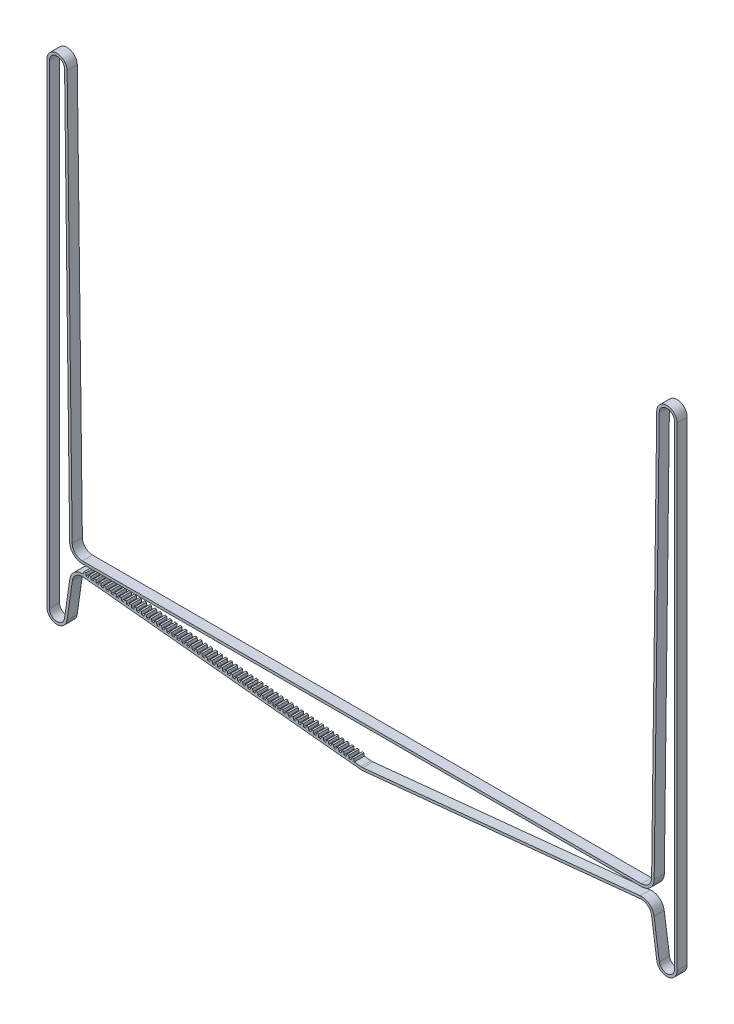
from build123d import *

# Parameters (mm, degrees)
BOSS_EXTRUDE1_DEPTH = 6
BOSS_EXTRUDE2_DEPTH = 6
LPATTERN1_COUNT     = 54
LPATTERN1_PITCH     = 3


with BuildPart() as part:
    # Sketch1 → Boss-Extrude1 (new body)
    with BuildSketch(Plane.XY):
        with BuildLine():
            Line((-136.619529898, -129.381794908), (27.031698215, -145.814248682))
            ThreePointArc((27.031698215, -145.814248682), (27.78101593, -145.851774363), (28.530333645, -145.814248682))
            Line((28.530333645, -145.814248682), (192.181561758, -129.381794908))
            ThreePointArc((192.181561758, -129.381794908), (196.478349535, -130.626340604), (198.719904672, -134.497607806))
            Line((198.719904672, -134.497607806), (201.842127188, -156.20594092))
            ThreePointArc((201.842127188, -156.20594092), (208.209190863, -161.336477048), (213.78101593, -155.351774363))
            Line((213.78101593, -155.351774363), (213.78101593, 124.648225637))
            ThreePointArc((213.78101593, 124.648225637), (207.818502024, 130.648108535), (201.781484333, 124.723196362))
            Line((201.781484333, 124.723196362), (198.780547528, -115.426745088))
            ThreePointArc((198.780547528, -115.426745088), (196.997067143, -119.620838918), (192.78101593, -121.351774363))
            Line((192.78101593, -121.351774363), (-137.21898407, -121.351774363))
            ThreePointArc((-137.21898407, -121.351774363), (-141.435035282, -119.620838918), (-143.218515667, -115.426745088))
            Line((-143.218515667, -115.426745088), (-146.219452472, 124.723196362))
            ThreePointArc((-146.219452472, 124.723196362), (-152.256470164, 130.648108535), (-158.21898407, 124.648225637))
            Line((-158.21898407, 124.648225637), (-158.21898407, -155.351774363))
            ThreePointArc((-158.21898407, -155.351774363), (-152.647159003, -161.336477048), (-146.280095328, -156.20594092))
            Line((-146.280095328, -156.20594092), (-143.157872812, -134.497607806))
            ThreePointArc((-143.157872812, -134.497607806), (-140.916317675, -130.626340604), (-136.619529898, -129.381794908))
        make_face()
        with BuildLine():
            Line((-136.469666355, -127.889300044), (27.181561758, -144.321753818))
            ThreePointArc((27.181561758, -144.321753818), (27.78101593, -144.351774363), (28.380470102, -144.321753818))
            Line((28.380470102, -144.321753818), (192.031698215, -127.889300044))
            ThreePointArc((192.031698215, -127.889300044), (197.402682936, -129.444982164), (200.204626858, -134.284066167))
            Line((200.204626858, -134.284066167), (203.326849373, -155.992399281))
            ThreePointArc((203.326849373, -155.992399281), (208.10214713, -159.840301377), (212.28101593, -155.351774363))
            Line((212.28101593, -155.351774363), (212.28101593, 124.648225637))
            ThreePointArc((212.28101593, 124.648225637), (207.809130501, 129.14813781), (203.281367232, 124.70445368))
            Line((203.281367232, 124.70445368), (200.280430427, -115.445487769))
            ThreePointArc((200.280430427, -115.445487769), (198.051079946, -120.688105057), (192.78101593, -122.851774363))
            Line((192.78101593, -122.851774363), (-137.21898407, -122.851774363))
            ThreePointArc((-137.21898407, -122.851774363), (-142.489048085, -120.688105057), (-144.718398567, -115.445487769))
            Line((-144.718398567, -115.445487769), (-147.719335372, 124.70445368))
            ThreePointArc((-147.719335372, 124.70445368), (-152.24709864, 129.14813781), (-156.71898407, 124.648225637))
            Line((-156.71898407, 124.648225637), (-156.71898407, -155.351774363))
            ThreePointArc((-156.71898407, -155.351774363), (-152.540115269, -159.840301377), (-147.764817513, -155.992399281))
            Line((-147.764817513, -155.992399281), (-144.642594998, -134.284066167))
            ThreePointArc((-144.642594998, -134.284066167), (-141.840651076, -129.444982164), (-136.469666355, -127.889300044))
        make_face(mode=Mode.SUBTRACT)
    extrude(amount=BOSS_EXTRUDE1_DEPTH)

    # Sketch2 → Boss-Extrude2 (add)
    with BuildSketch(Plane.XY.offset(6)):
        Polygon((22.954875191, -142.389803301), (21.959878615, -142.289894273), (21.410102278, -143.742233321), (23.204924441, -143.92245398), align=None)
    boss_extrude2 = extrude(amount=-BOSS_EXTRUDE2_DEPTH)

    # LPattern1: Boss-Extrude2 ×54
    with Locations(*[Vector(-0.9949965758703774, 0.09990902865219185, 0) * (i * LPATTERN1_PITCH) for i in range(1, LPATTERN1_COUNT)]):
        add(boss_extrude2)


solid = part.part
